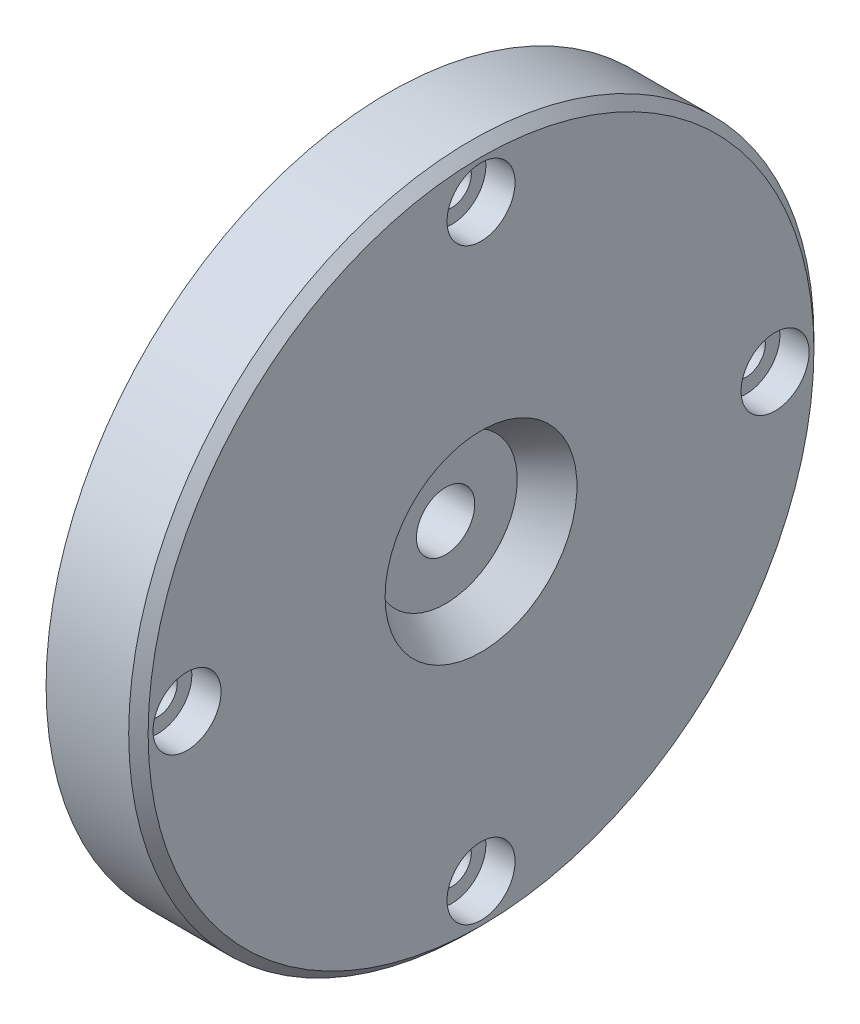
from build123d import *

# Parameters (mm, degrees)
CHAMFER1_SIZE      = 2
SKETCH2_R          = 4
CUT_EXTRUDE1_DEPTH = 49
SKETCH3_R          = 7
CUT_EXTRUDE2_DEPTH = 6


with BuildPart() as part:
    # Sketch1 → Revolve1 (revolve)
    with BuildSketch(Plane.XY, mode=Mode.PRIVATE) as revolve1_sk:
        Polygon((-28.741506647, 6), (-28.741506647, 51.5), (-21.741506647, 51.5), (-21.741506647, 70.5), (-2.741506647, 70.5), (-2.741506647, 19.745937962), (-10.031019202, 14.747415066), (-10.031019202, 6), align=None)
    revolve(revolve1_sk.sketch.rotate(Axis((-75.394387001, 0, 0), (1, 0, 0)), 90), axis=Axis((-75.394387001, 0, 0), (1, 0, 0)))

    # Chamfer1
    chamfer1_edges = [part.edges().sort_by_distance(p)[0] for p in [
        (-2.741506647, 0, -70.5),
    ]]
    chamfer(chamfer1_edges, length=CHAMFER1_SIZE)

    # Sketch2 → Cut-Extrude1 (cut)
    with BuildSketch(Plane(origin=(-2.741506647, 0, 0), x_dir=(0, 0, -1), z_dir=(1, 0, 0))):
        with Locations((0, -60.5)):
            Circle(SKETCH2_R)
        with Locations((-60.5, 0)):
            Circle(SKETCH2_R)
        with Locations((0, 60.5)):
            Circle(SKETCH2_R)
        with Locations((60.5, 0)):
            Circle(SKETCH2_R)
    extrude(amount=-CUT_EXTRUDE1_DEPTH, mode=Mode.SUBTRACT)

    # Sketch3 → Cut-Extrude2 (cut)
    with BuildSketch(Plane(origin=(-2.741506647, 0, 0), x_dir=(0, 0, -1), z_dir=(1, 0, 0))):
        with Locations((-60.5, 0)):
            Circle(SKETCH3_R)
        with Locations((0, 60.5)):
            Circle(SKETCH3_R)
        with Locations((60.5, 0)):
            Circle(SKETCH3_R)
        with Locations((0, -60.5)):
            Circle(SKETCH3_R)
    extrude(amount=-CUT_EXTRUDE2_DEPTH, mode=Mode.SUBTRACT)


solid = part.part
